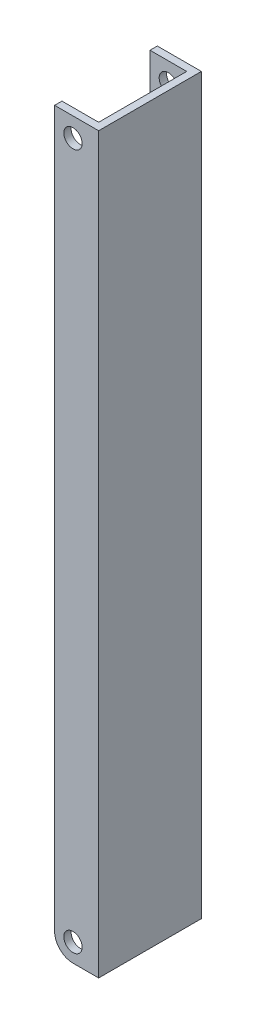
SolidWorks part; units mm, degrees
ref_plane "Front Plane" through (0, 0, 0) normal (0, 0, 1) x (1, 0, 0)
ref_plane "Top Plane" through (0, 0, 0) normal (0, 1, 0) x (1, 0, 0)
ref_plane "Right Plane" through (0, 0, 0) normal (1, 0, 0) x (0, 0, -1)
other "Configuration Table"
ref_plane "Plane1" through (0, 50, 0) normal (0, 1, 0) x (1, 0, 0)
sketch "Sketch2" plane through (0, 50, 0) normal (0, 1, 0) x (1, 0, 0)
  line L5 (27, 22) -> (37, 22)
  line L6 (37, 22) -> (37, -2)
  line L7 (37, -2) -> (27, -2)
  line L11 (27, 24) -> (39, 24)
  line L12 (39, 24) -> (39, -4)
  line L13 (39, -4) -> (27, -4)
  line L20 (27, 22) -> (27, 24)
  line L21 (27, -2) -> (27, -4)
  line L22 (39, -4) -> (25, -4) construction
  line L23 (25, -4) -> (25, 2) construction
  line L24 (27, -2) -> (27, 0) construction
  line L25 (27, 0) -> (35, 0) construction
  line L26 (25, 2) -> (33, 2) construction
  line L27 (33, 2) -> (33, 10) construction
  line L28 (35, 0) -> (35, 10) construction
  line L29 (33, 10) -> (33, 18) construction
  line L30 (35, 10) -> (35, 20) construction
  line L31 (35, 20) -> (27, 20) construction
  line L32 (33, 18) -> (25, 18) construction
  line L33 (27, 20) -> (27, 22) construction
  line L34 (25, 18) -> (25, 24) construction
  line L35 (25, 24) -> (39, 24) construction
  dimension "D1" = 28
  dimension "D2" = 12
  dimension "D3" = 10
  dimension "D5" = 2
extrude "Boss-Extrude1" add sketch "Sketch2" along normal blind 200
fillet "Fillet1" radius 5 2 edges at (27, 50, 3) (27, 50, -23)
sketch "Sketch3" plane through (0, 0, 2) normal (0, 0, -1) x (-1, 0, 0)
  circle A0 centre (-32, 55) radius 2.5
  dimension "D1" = 5
extrude "Cut-Extrude1" cut sketch "Sketch3" against normal through all both and the other way through all
sketch "Sketch9" plane through (0, 0, -22) normal (0, 0, -1) x (-1, 0, 0)
  circle A0 centre (-32, 244.7301) radius 2.5
  dimension "D1" = 5
extrude "Cut-Extrude2" cut sketch "Sketch9" against normal through all both and the other way through all
